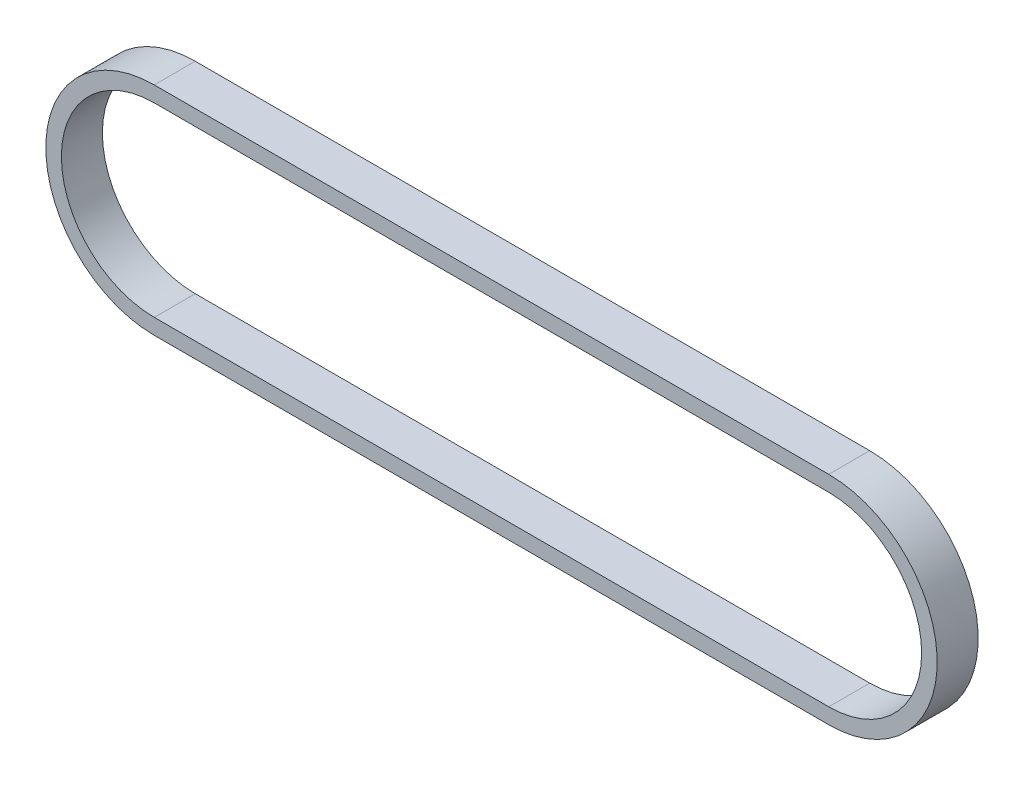
from build123d import *

# Parameters (mm, degrees)
BOSS_EXTRUDE1_DEPTH = 7.9
SHELL1_T            = -3


with BuildPart() as part:
    # Sketch2 → Boss-Extrude1 (new body)
    with BuildSketch(Plane.XY):
        with BuildLine():
            Line((0, 20.9), (-130, 20.9))
            ThreePointArc((-130, 20.9), (-150.9, 0), (-130, -20.9))
            Line((-130, -20.9), (0, -20.9))
            ThreePointArc((0, -20.9), (20.9, 0), (0, 20.9))
        make_face()
    extrude(amount=BOSS_EXTRUDE1_DEPTH)

    # Shell1
    shell1_openings = [part.faces().sort_by_distance(p)[0] for p in [
        (-65, 0, 7.9),
        (-65, 0, 0),
    ]]
    offset(amount=SHELL1_T, openings=shell1_openings, kind=Kind.INTERSECTION)


solid = part.part
